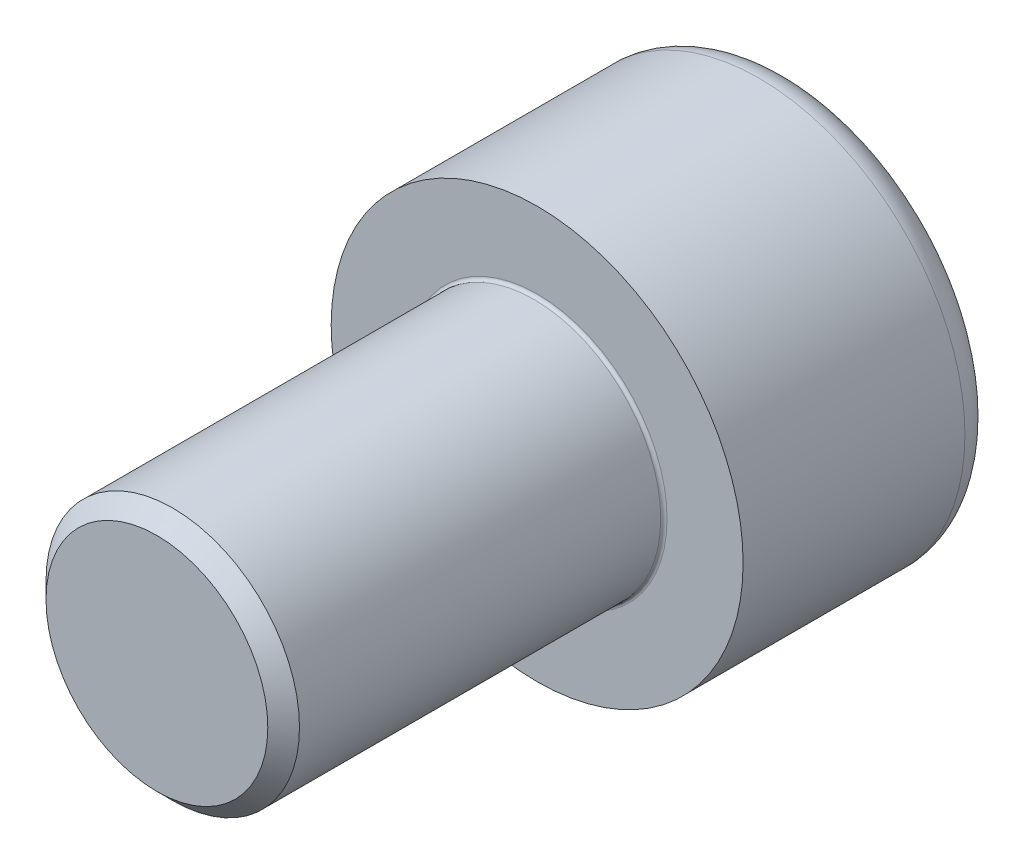
from build123d import *

# Parameters (mm, degrees)
SKETCH_1_R          = 6.5
EXTRUDE_1_DEPTH     = 8
SKETCH_2_R          = 4
EXTRUDE_2_DEPTH     = 12
CUT_EXTRUDE_1_DEPTH = 4
FILLET_1_R          = 0.1
CHAMFER_1_SIZE      = 0.5
FILLET_2_R          = 1


with BuildPart() as part:
    # 草图1 → 凸台-拉伸1 (new body)
    with BuildSketch(Plane.XY):
        Circle(SKETCH_1_R)
    extrude(amount=EXTRUDE_1_DEPTH)

    # 草图2 → 凸台-拉伸2 (add)
    with BuildSketch(Plane.XY.offset(8)):
        Circle(SKETCH_2_R)
    extrude(amount=EXTRUDE_2_DEPTH)

    # 草图3 → 切除-拉伸1 (cut)
    with BuildSketch(Plane(origin=(0, 0, 0), x_dir=(-1, 0, 0), z_dir=(0, 0, -1))):
        Polygon((1.732050808, -3), (3.464101615, 0), (1.732050808, 3), (-1.732050808, 3), (-3.464101615, 0), (-1.732050808, -3), align=None)
    extrude(amount=-CUT_EXTRUDE_1_DEPTH, mode=Mode.SUBTRACT)

    # 圆角1
    fillet_1_edges = [part.edges().sort_by_distance(p)[0] for p in [
        (-4, 0, 8),
    ]]
    fillet(fillet_1_edges, radius=FILLET_1_R)

    # 倒角1
    chamfer_1_edges = [part.edges().sort_by_distance(p)[0] for p in [
        (-4, 0, 20),
    ]]
    chamfer(chamfer_1_edges, length=CHAMFER_1_SIZE)

    # 圆角2
    fillet_2_edges = [part.edges().sort_by_distance(p)[0] for p in [
        (-6.5, 0, 0),
    ]]
    fillet(fillet_2_edges, radius=FILLET_2_R)


solid = part.part
